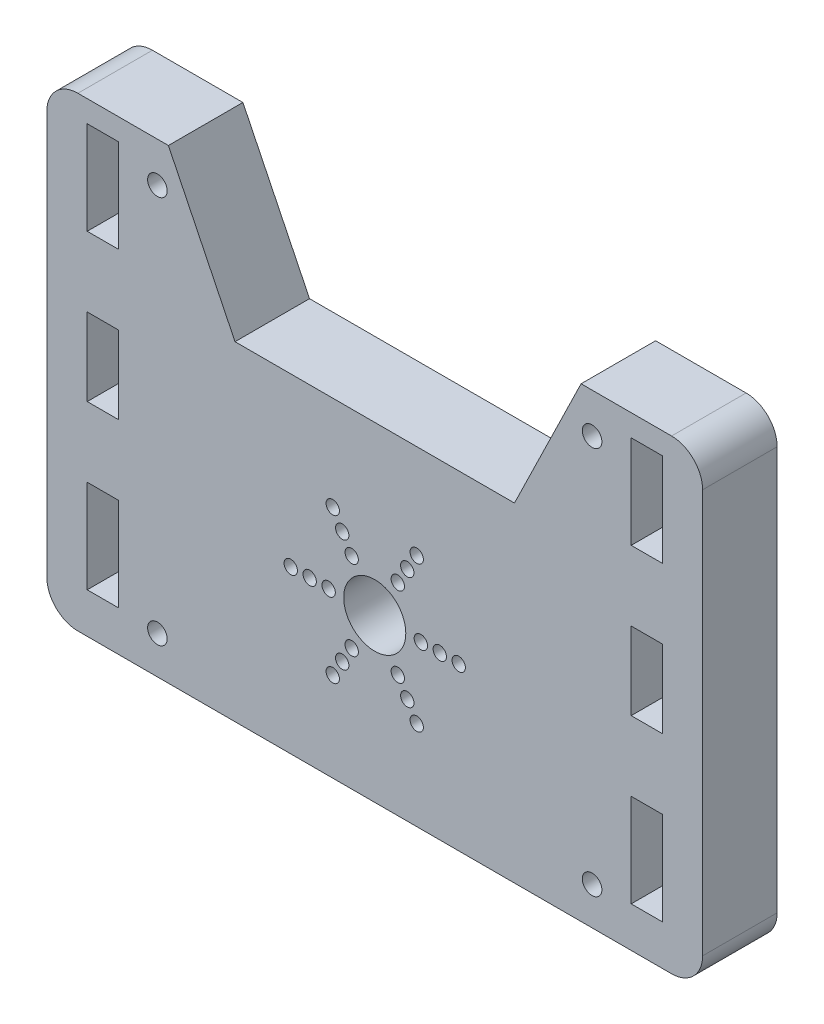
from build123d import *

# Parameters (mm, degrees)
SKETCH_1_R      = 1.575
SKETCH_1_R_2    = 5
SKETCH_1_R_3    = 1.075
SKETCH_1_W      = 5
SKETCH_1_H      = 15
SKETCH_1_H_2    = 12.5
EXTRUDE_1_DEPTH = 12


with BuildPart() as part:
    # 草图1 → 凸台-拉伸1 (new body)
    with BuildSketch(Plane.XY):
        with BuildLine():
            Line((-33.144127259, 37.474667316), (-22.414010311, 15.474667316))
            Line((-22.414010311, 15.474667316), (22.585989689, 15.474667316))
            Line((22.585989689, 15.474667316), (33.316106638, 37.474667316))
            Line((33.316106638, 37.474667316), (47.885989689, 37.474667316))
            ThreePointArc((47.885989689, 37.474667316), (51.421523595, 36.010201222), (52.885989689, 32.474667316))
            Line((52.885989689, 32.474667316), (52.885989689, -32.525332684))
            ThreePointArc((52.885989689, -32.525332684), (51.421523595, -36.060866589), (47.885989689, -37.525332684))
            Line((47.885989689, -37.525332684), (-47.714010311, -37.525332684))
            ThreePointArc((-47.714010311, -37.525332684), (-51.249544217, -36.060866589), (-52.714010311, -32.525332684))
            Line((-52.714010311, -32.525332684), (-52.714010311, 32.474667316))
            ThreePointArc((-52.714010311, 32.474667316), (-51.249544217, 36.010201222), (-47.714010311, 37.474667316))
            Line((-47.714010311, 37.474667316), (-33.144127259, 37.474667316))
        make_face()
        with Locations((35.085989689, 31.055295289)):
            Circle(SKETCH_1_R, mode=Mode.SUBTRACT)
        with Locations((35.085989689, -31.444704711)):
            Circle(SKETCH_1_R, mode=Mode.SUBTRACT)
        with Locations((0.085989689, -11.444704711)):
            Circle(SKETCH_1_R_2, mode=Mode.SUBTRACT)
        with Locations((7.510989689, -11.444704711)):
            Circle(SKETCH_1_R_3, mode=Mode.SUBTRACT)
        with Locations((10.560989689, -11.444704711)):
            Circle(SKETCH_1_R_3, mode=Mode.SUBTRACT)
        with Locations((13.610989689, -11.444704711)):
            Circle(SKETCH_1_R_3, mode=Mode.SUBTRACT)
        with Locations((5.323489689, -20.516320815)):
            Circle(SKETCH_1_R_3, mode=Mode.SUBTRACT)
        with Locations((3.798489689, -17.874943334)):
            Circle(SKETCH_1_R_3, mode=Mode.SUBTRACT)
        with Locations((6.848489689, -23.157698297)):
            Circle(SKETCH_1_R_3, mode=Mode.SUBTRACT)
        with Locations((-5.151510311, -20.516320815)):
            Circle(SKETCH_1_R_3, mode=Mode.SUBTRACT)
        with Locations((-3.626510311, -17.874943334)):
            Circle(SKETCH_1_R_3, mode=Mode.SUBTRACT)
        with Locations((-6.676510311, -23.157698297)):
            Circle(SKETCH_1_R_3, mode=Mode.SUBTRACT)
        with Locations((-10.389010311, -11.444704711)):
            Circle(SKETCH_1_R_3, mode=Mode.SUBTRACT)
        with Locations((-7.339010311, -11.444704711)):
            Circle(SKETCH_1_R_3, mode=Mode.SUBTRACT)
        with Locations((-13.439010311, -11.444704711)):
            Circle(SKETCH_1_R_3, mode=Mode.SUBTRACT)
        with Locations((-5.151510311, -2.373088606)):
            Circle(SKETCH_1_R_3, mode=Mode.SUBTRACT)
        with Locations((-3.626510311, -5.014466088)):
            Circle(SKETCH_1_R_3, mode=Mode.SUBTRACT)
        with Locations((-6.676510311, 0.268288875)):
            Circle(SKETCH_1_R_3, mode=Mode.SUBTRACT)
        with Locations((5.323489689, -2.373088606)):
            Circle(SKETCH_1_R_3, mode=Mode.SUBTRACT)
        with Locations((3.798489689, -5.014466088)):
            Circle(SKETCH_1_R_3, mode=Mode.SUBTRACT)
        with Locations((6.848489689, 0.268288875)):
            Circle(SKETCH_1_R_3, mode=Mode.SUBTRACT)
        with Locations(Location((-34.914010311, 31.055295289, 0), (0, 0, 180))):
            Circle(SKETCH_1_R, mode=Mode.SUBTRACT)
        with Locations(Location((-34.914010311, -31.444704711, 0), (0, 0, 180))):
            Circle(SKETCH_1_R, mode=Mode.SUBTRACT)
        with Locations((-43.714010311, -23.525332684)):
            Rectangle(SKETCH_1_W, SKETCH_1_H, mode=Mode.SUBTRACT)
        with Locations((43.885989689, -23.525332684)):
            Rectangle(SKETCH_1_W, SKETCH_1_H, mode=Mode.SUBTRACT)
        with Locations((43.885989689, 1.474667316)):
            Rectangle(SKETCH_1_W, SKETCH_1_H_2, mode=Mode.SUBTRACT)
        with Locations((43.885989689, 26.474667316)):
            Rectangle(SKETCH_1_W, SKETCH_1_H, mode=Mode.SUBTRACT)
        with Locations((-43.714010311, 1.474667316)):
            Rectangle(SKETCH_1_W, SKETCH_1_H_2, mode=Mode.SUBTRACT)
        with Locations((-43.714010311, 26.474667316)):
            Rectangle(SKETCH_1_W, SKETCH_1_H, mode=Mode.SUBTRACT)
    extrude(amount=EXTRUDE_1_DEPTH)


solid = part.part
